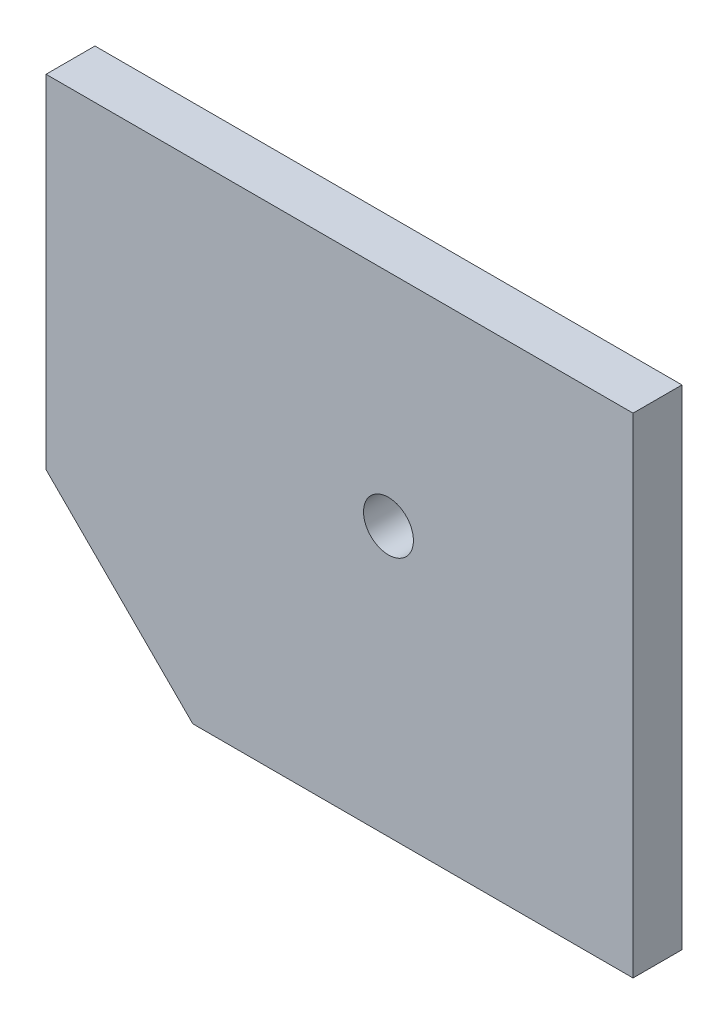
SolidWorks part; units mm, degrees
ref_plane "前视基准面" through (0, 0, 0) normal (0, 0, 1) x (1, 0, 0)
ref_plane "上视基准面" through (0, 0, 0) normal (0, 1, 0) x (1, 0, 0)
ref_plane "右视基准面" through (0, 0, 0) normal (1, 0, 0) x (0, 0, -1)
sketch "草图1" plane through (0, 0, 0) normal (0, 0, 1) x (1, 0, 0)
  line L0 (-30.8451, -49.2958) -> (-60.8451, -19.2958)
  line L1 (-60.8451, 50.7042) -> (59.1549, 50.7042)
  line L2 (-60.8451, 50.7042) -> (-60.8451, -19.2958)
  line L3 (-30.8451, -49.2958) -> (59.1549, -49.2958)
  line L4 (59.1549, 50.7042) -> (59.1549, -49.2958)
  line L5 (-60.8451, 50.7042) -> (59.1549, -49.2958) construction
  line L6 (-43.1528, -36.9881) -> (59.1549, 50.7042) construction
  point P0 (0, 0)
  dimension "D1" = 120
  dimension "D2" = 100
  dimension "D3" = 90
  dimension "D4" = 70
extrude "凸台-拉伸1" add sketch "草图1" along normal blind 10
hole_wizard "M12 螺纹孔1" positions "草图3" profile "草图2" tap size "M12" standard "Gb"
sketch "草图3" plane through (0, 0, 10) normal (0, 0, 1) x (1, 0, 0)
  line L0 (-60.8451, 50.7042) -> (-60.8451, -19.2958) construction
  line L1 (-30.8451, -49.2958) -> (59.1549, -49.2958) construction
  point P0 (9.1549, 5.7042)
  dimension "D1" = 70
  dimension "D2" = 55
sketch "草图2" plane through (9.1549, 5.7042, 10) normal (1, 0, 0) x (0, -1, 0)
  line L0 (0, 0) -> (0, 35.8144)
  line L1 (0, 35.8144) -> (5.1, 32.75)
  line L2 (5.1, 32.75) -> (5.1, 0)
  line L5 (5.1, 0) -> (0, 0)
  line L10 (0, 35.8144) -> (-5.1, 32.75) construction
  line L11 (0, -6.35) -> (0, 107.95) construction
  dimension "螺纹孔钻头直径" = 10.2
  dimension "螺纹孔钻头深度" = 32.75
  dimension "导头角度" = 118
cosmetic thread "孔螺蚊线1" parameters "D1"=8, "D2"=12
